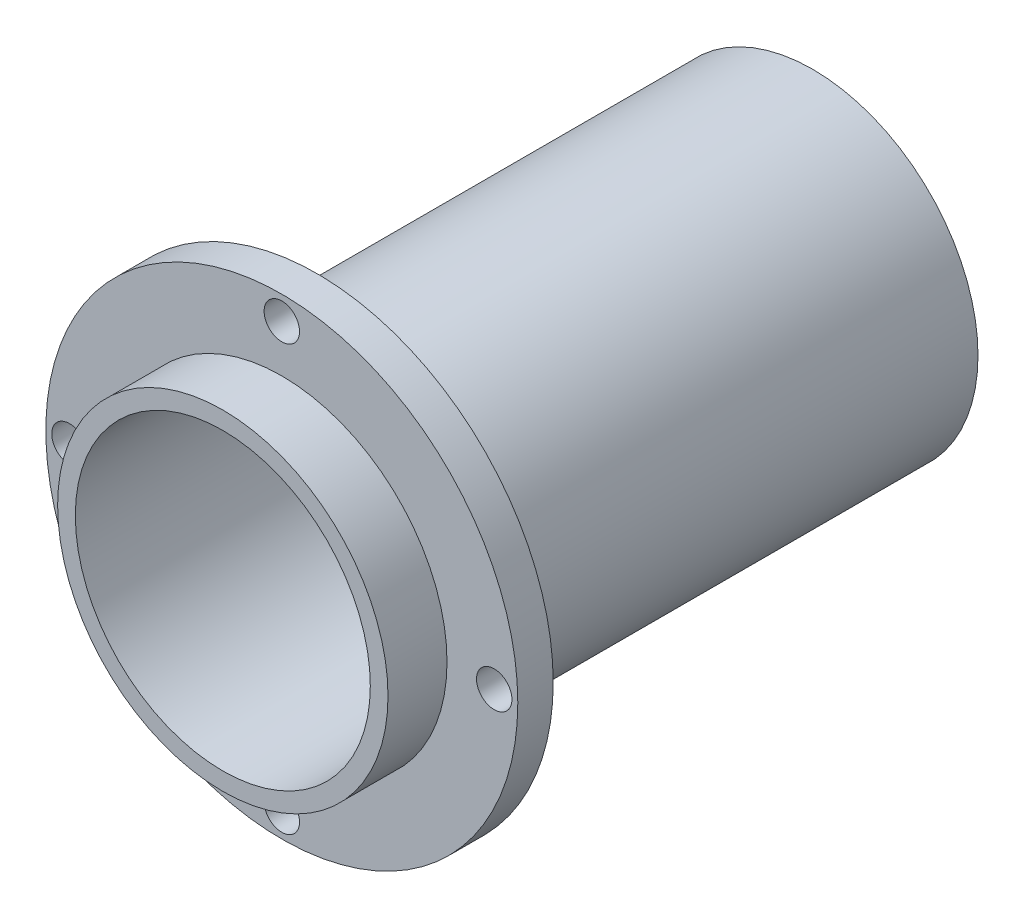
from build123d import *

# Parameters (mm, degrees)
SKETCH1_R           = 14
SKETCH1_R_2         = 12.5
BOSS_EXTRUDE1_DEPTH = 25
BOSS_EXTRUDE2_START = -8
SKETCH2_R           = 20
SKETCH2_R_2         = 1.5
SKETCH2_R_3         = 12.5
BOSS_EXTRUDE2_DEPTH = 3


with BuildPart() as part:
    # Sketch1 → Boss-Extrude1 (new, symmetric)
    with BuildSketch(Plane.XY):
        Circle(SKETCH1_R)
        Circle(SKETCH1_R_2, mode=Mode.SUBTRACT)
    extrude(amount=BOSS_EXTRUDE1_DEPTH, both=True)

    # Sketch2 → Boss-Extrude2 (add)
    with BuildSketch(Plane.XY.offset(25).offset(BOSS_EXTRUDE2_START)):
        Circle(SKETCH2_R)
        with Locations((0, 18)):
            Circle(SKETCH2_R_2, mode=Mode.SUBTRACT)
        with Locations((18, 0)):
            Circle(SKETCH2_R_2, mode=Mode.SUBTRACT)
        with Locations((0, -18)):
            Circle(SKETCH2_R_2, mode=Mode.SUBTRACT)
        with Locations((-18, 0)):
            Circle(SKETCH2_R_2, mode=Mode.SUBTRACT)
        Circle(SKETCH2_R_3, mode=Mode.SUBTRACT)
    extrude(amount=BOSS_EXTRUDE2_DEPTH)


solid = part.part
